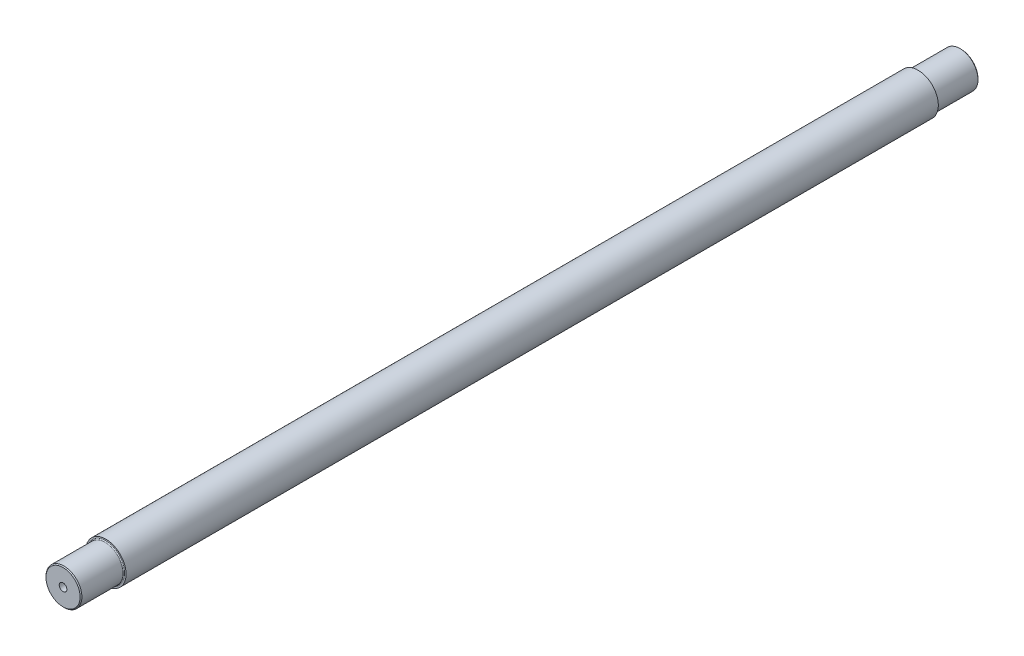
from build123d import *

# Parameters (mm, degrees)
SKETCH_1_R              = 22.5
EXTRUDE_1_DEPTH         = 904.6
SKETCH_2_R              = 20
EXTRUDE_2_DEPTH         = 47.7
EXTRUDE_START           = 47.7
SKETCH_3_R              = 20
EXTRUDE_3_DEPTH         = 47.7
FILLET_1_R              = 1
CHAMFER_1_SIZE          = 1
HOLE_WIZARD_M10_1_D     = 8.5
HOLE_WIZARD_M10_1_DEPTH = 24.5
HOLE_WIZARD_M10_1_TIP   = 2.553657631
HOLE_WIZARD_M10_2_D     = 8.5
HOLE_WIZARD_M10_2_DEPTH = 24.5
HOLE_WIZARD_M10_2_TIP   = 2.553657631


with BuildPart() as part:
    # 草图1 → 凸台-拉伸1 (new body)
    with BuildSketch(Plane.XY):
        with Locations(Location((0, 0, 0), (0, 0, 180))):
            Circle(SKETCH_1_R)
    extrude(amount=EXTRUDE_1_DEPTH)

    # 草图2 → 凸台-拉伸2 (add)
    with BuildSketch(Plane.XY.offset(904.6)):
        Circle(SKETCH_2_R)
    extrude(amount=EXTRUDE_2_DEPTH)

    # 草图3 → 凸台-拉伸3 (add)
    with BuildSketch(Plane(origin=(0, 0, 0), x_dir=(-1, 0, 0), z_dir=(0, 0, -1)).offset(EXTRUDE_START)):
        with Locations(Location((0, 0, 0), (0, 0, 180))):
            Circle(SKETCH_3_R)
    extrude(amount=-EXTRUDE_3_DEPTH)

    # 圆角1
    fillet_1_edges = [part.edges().sort_by_distance(p)[0] for p in [
        (-20, 0, 904.6),
        (-20, 0, 0),
    ]]
    fillet(fillet_1_edges, radius=FILLET_1_R)

    # 倒角1
    chamfer_1_edges = [part.edges().sort_by_distance(p)[0] for p in [
        (-20, 0, -47.7),
        (-20, 0, 952.3),
    ]]
    chamfer(chamfer_1_edges, length=CHAMFER_1_SIZE)

    # M10 螺纹孔1
    with Locations(Plane.XY.offset(952.3)):
        with Locations((0, 0)):
            Hole(HOLE_WIZARD_M10_1_D / 2, depth=HOLE_WIZARD_M10_1_DEPTH)
            with Locations((0, 0, -(HOLE_WIZARD_M10_1_DEPTH + HOLE_WIZARD_M10_1_TIP / 2))):  # 118° drill point
                Cone(0, HOLE_WIZARD_M10_1_D / 2, HOLE_WIZARD_M10_1_TIP, mode=Mode.SUBTRACT)

    # M10 螺纹孔2
    with Locations(Plane(origin=(0, 0, -47.7), x_dir=(-1, 0, 0), z_dir=(0, 0, -1))):
        with Locations((0, 0)):
            Hole(HOLE_WIZARD_M10_2_D / 2, depth=HOLE_WIZARD_M10_2_DEPTH)
            with Locations((0, 0, -(HOLE_WIZARD_M10_2_DEPTH + HOLE_WIZARD_M10_2_TIP / 2))):  # 118° drill point
                Cone(0, HOLE_WIZARD_M10_2_D / 2, HOLE_WIZARD_M10_2_TIP, mode=Mode.SUBTRACT)


solid = part.part
